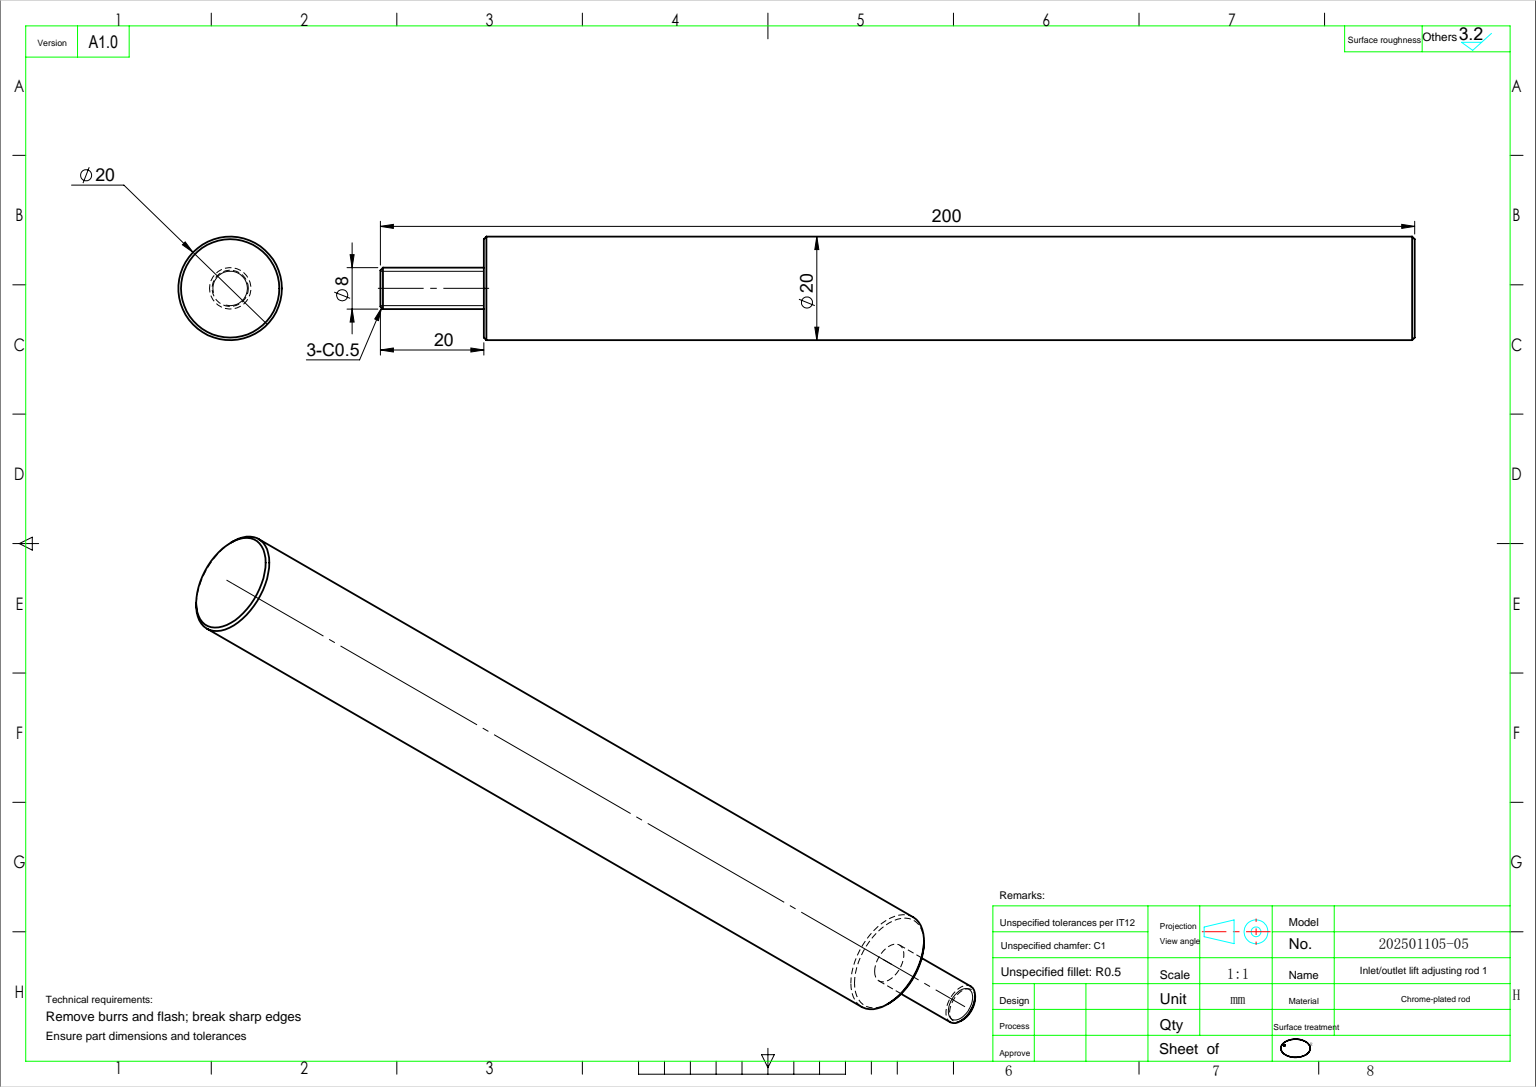
SolidWorks part; units mm, degrees
ref_plane "前视基准面" through (0, 0, 0) normal (0, 0, 1) x (1, 0, 0)
ref_plane "上视基准面" through (0, 0, 0) normal (0, 1, 0) x (1, 0, 0)
ref_plane "右视基准面" through (0, 0, 0) normal (1, 0, 0) x (0, 0, -1)
sketch "草图1" plane through (0, 0, 0) normal (0, 0, 1) x (1, 0, 0)
  circle A0 centre (0, 0) radius 10
  dimension "D1" = 20
extrude "凸台-拉伸1" add sketch "草图1" along normal blind 200
sketch "草图2" plane through (0, 0, 0) normal (0, 0, -1) x (-1, 0, 0)
  circle A0 centre (0, 0) radius 4
  dimension "D1" = 8
extrude "切除-拉伸1" cut sketch "草图2" against normal blind 20 flip side to cut
cosmetic thread "装饰螺纹线1" parameters "D2"=6.647
chamfer "倒角1" distance 0.5 angle 45 3 edges at (-10, 0, 20) (10, 0, 200) (-4, 0, 0)
